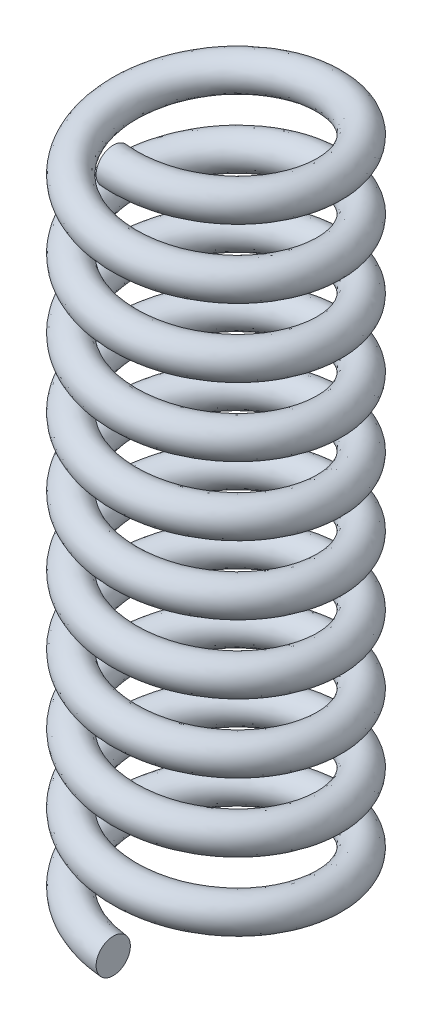
SolidWorks part; units mm, degrees
material "1060 Alloy"
ref_plane "Front Plane" through (0, 0, 0) normal (0, 0, 1) x (1, 0, 0)
ref_plane "Top Plane" through (0, 0, 0) normal (0, 1, 0) x (1, 0, 0)
ref_plane "Right Plane" through (0, 0, 0) normal (1, 0, 0) x (0, 0, -1)
sketch "Sketch1" plane through (0, 0, 0) normal (0, 0, 1) x (1, 0, 0)
  circle A0 centre (3, 0) radius 0.5
  dimension "D2" = 1
  dimension "D1" = 3
sketch "Sketch3" plane through (0, 0, 0) normal (0, 1, 0) x (1, 0, 0)
  circle A0 centre (0, 0) radius 3
  dimension "D1" = 6
curve "Helix/Spiral1" pitch 2 height 20 turns 10
sweep "Sweep1" add profiles "Sketch1" path "Helix/Spiral1"
